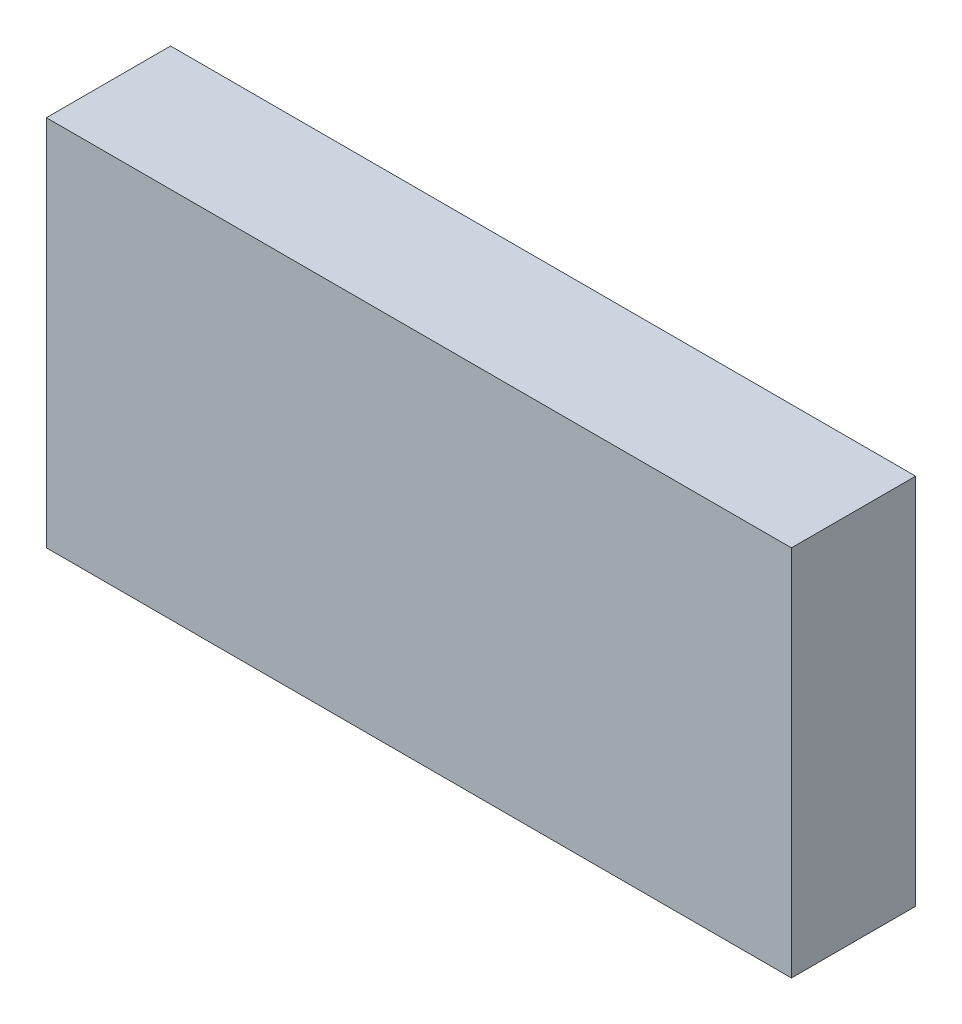
from build123d import *

# Parameters (mm, degrees)
SKETCH1_W           = 120
SKETCH1_H           = 60
BOSS_EXTRUDE1_DEPTH = 20


with BuildPart() as part:
    # Sketch1 → Boss-Extrude1 (new body)
    with BuildSketch(Plane.XY):
        with Locations((60, 30)):
            Rectangle(SKETCH1_W, SKETCH1_H)
    extrude(amount=BOSS_EXTRUDE1_DEPTH)


solid = part.part
